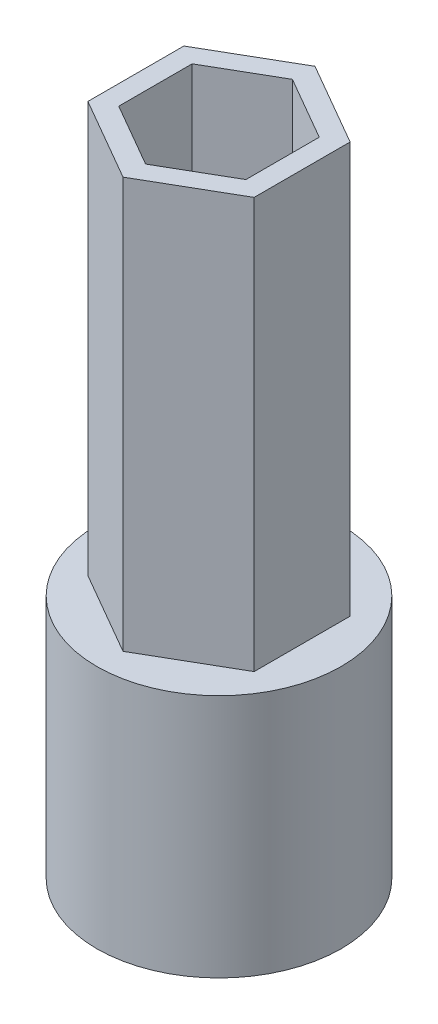
from build123d import *

# Parameters (mm, degrees)
BOSS_EXTRUDE3_DEPTH = 5
BOSS_EXTRUDE4_DEPTH = 8.4
SHELL1_T            = -0.4


with BuildPart() as part:
    # Sketch1 → Boss-Extrude3 (new body)
    with BuildSketch(Plane(origin=(0, 0, 0), x_dir=(1, 0, 0), z_dir=(0, 1, 0))):
        with BuildLine():
            ThreePointArc((0, 2.5), (-1.25, 2.165063509), (-2.165063509, 1.25))
            ThreePointArc((-2.165063509, 1.25), (-2.5, 0), (-2.165063509, -1.25))
            ThreePointArc((-2.165063509, -1.25), (-1.25, -2.165063509), (0, -2.5))
            ThreePointArc((0, -2.5), (1.25, -2.165063509), (2.165063509, -1.25))
            ThreePointArc((2.165063509, -1.25), (2.5, 0), (2.165063509, 1.25))
            ThreePointArc((2.165063509, 1.25), (1.25, 2.165063509), (0, 2.5))
        make_face()
    extrude(amount=BOSS_EXTRUDE3_DEPTH)

    # Sketch2 → Boss-Extrude4 (add)
    with BuildSketch(Plane(origin=(0, 13.4, 0), x_dir=(1, 0, 0), z_dir=(0, 1, 0))):
        Polygon((0, 1.962990915), (-1.7, 0.981495458), (-1.7, -0.981495458), (0, -1.962990915), (1.7, -0.981495458), (1.7, 0.981495458), align=None)
    extrude(amount=-BOSS_EXTRUDE4_DEPTH)

    # Shell1
    shell1_openings = [part.faces().sort_by_distance(p)[0] for p in [
        (0, 13.4, 0),
        (0, 0, 0),
    ]]
    offset(amount=SHELL1_T, openings=shell1_openings, kind=Kind.INTERSECTION)


solid = part.part
